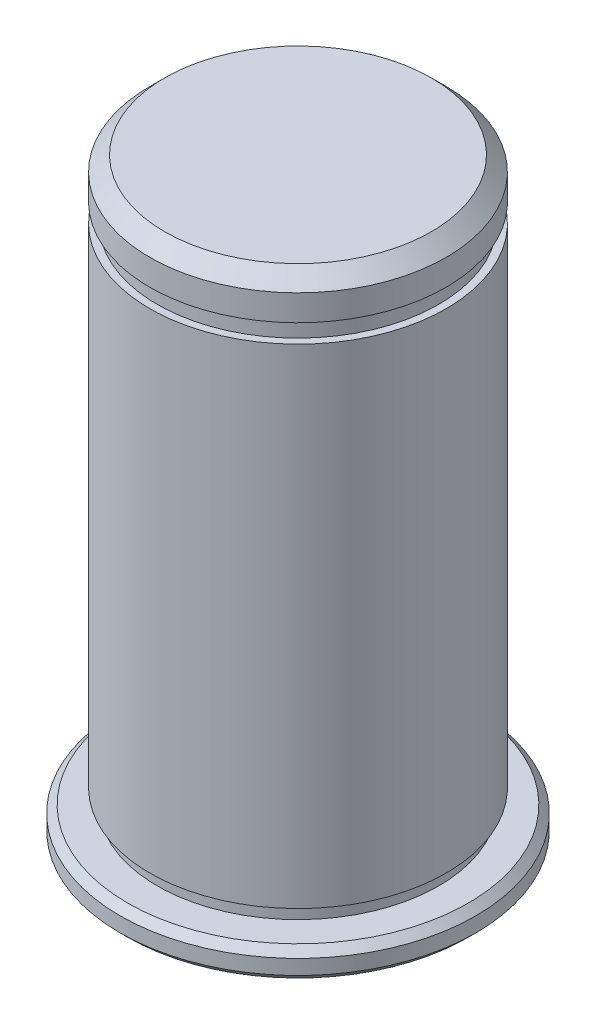
from build123d import *


with BuildPart() as part:
    # 草图1 → 旋转1 (revolve)
    with BuildSketch(Plane.XY, mode=Mode.PRIVATE) as revolve_1_sk:
        Polygon((11.5, 2), (9.5, 2), (9.5, 3), (10, 3), (10, 36), (9.5, 36), (9.5, 37.25), (10, 37.25), (10, 39), (9, 40), (0, 40), (0, 0), (11.5, 0), (12, 0.5), (12, 1.5), align=None)
    revolve(revolve_1_sk.sketch.rotate(Axis((0, -1.467272455, 0), (0, 1, 0)), 90), axis=Axis((0, -1.467272455, 0), (0, 1, 0)))


solid = part.part
